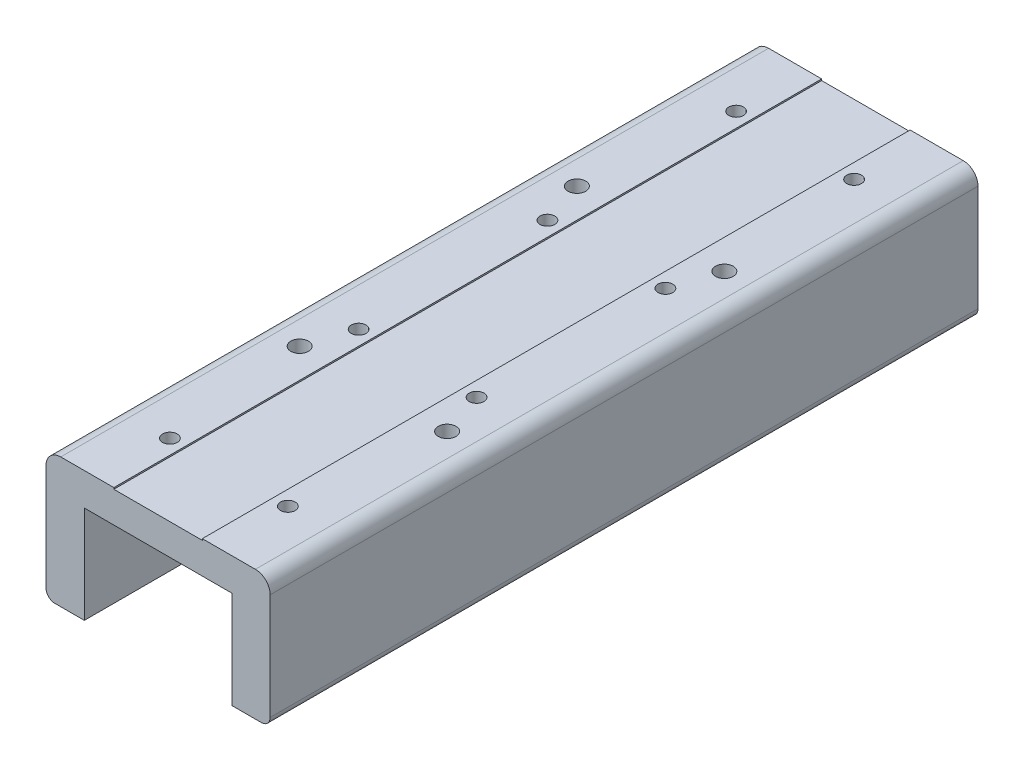
SolidWorks part; units mm, degrees
ref_plane "前视" through (0, 0, 0) normal (0, 0, 1) x (1, 0, 0)
ref_plane "上视" through (0, 0, 0) normal (0, 1, 0) x (1, 0, 0)
ref_plane "右视" through (0, 0, 0) normal (1, 0, 0) x (0, 0, -1)
sketch "草图1" plane through (0, 0, 0) normal (0, 0, 1) x (1, 0, 0)
  line L0 (0, 0) -> (0, 102.5797) construction
  line L1 (33, 50.7854) -> (15, 50.7854)
  line L2 (-38, 45.7854) -> (-38, 9.7854)
  line L3 (-35, 6.7854) -> (-25, 6.7854)
  line L4 (-25, 6.7854) -> (-25, 39.7854)
  line L5 (-25, 39.7854) -> (25, 39.7854)
  line L6 (25, 6.7854) -> (25, 39.7854)
  line L7 (35, 6.7854) -> (25, 6.7854)
  line L8 (38, 45.7854) -> (38, 9.7854)
  line L9 (-15, 50.7854) -> (-15, 50.2854)
  line L10 (-15, 50.2854) -> (15, 50.2854)
  line L11 (15, 50.7854) -> (15, 50.2854)
  line L12 (-15, 50.7854) -> (-33, 50.7854)
  arc A0 (-35, 6.7854) -> (-38, 9.7854) centre (-35, 9.7854) cw
  arc A1 (38, 9.7854) -> (35, 6.7854) centre (35, 9.7854) cw
  arc A2 (-38, 45.7854) -> (-33, 50.7854) centre (-33, 45.7854) cw
  arc A3 (38, 45.7854) -> (33, 50.7854) centre (33, 45.7854) ccw
  point P10 (0, 39.7854)
  point P13 (0, 50.7854)
  point P17 (0, 50.2854)
  point P20 (-38, 6.7854)
  point P23 (38, 6.7854)
  point P26 (-38, 50.7854)
  point P29 (38, 50.7854)
  dimension "D7" = 3
  dimension "D8" = 5
  dimension "D1" = 11
  dimension "D2" = 13
  dimension "D3" = 44
  dimension "D4" = 38
  dimension "D5" = 0.5
  dimension "D6" = 15
extrude "基体-拉伸" add sketch "草图1" against normal blind 240
ref_plane "基准面1" through (0, 0, -70) normal (0, 0, 1) x (1, 0, 0)
sketch "草图3" plane through (0, 50.7854, 0) normal (0, 1, 0) x (-1, 0, 0)
  line L0 (24.2, 0) -> (-24.2, 0) construction
  line L1 (-38, -240) -> (-38, 0) construction
  line L2 (-20, -24) -> (20, -24) construction
  line L3 (-20, -24) -> (-20, -88) construction
  line L4 (-25, -73) -> (25, -73) construction
  line L5 (-25, -73) -> (-25, -167) construction
  circle A0 centre (-20, -24) radius 2.5
  circle A1 centre (20, -24) radius 2.5
  circle A2 centre (-20, -88) radius 2.5
  circle A3 centre (20, -88) radius 2.5
  circle A4 centre (-20, -152) radius 2.5
  circle A5 centre (20, -152) radius 2.5
  circle A6 centre (-20, -216) radius 2.5
  circle A7 centre (20, -216) radius 2.5
  circle A8 centre (-25, -73) radius 3
  circle A9 centre (25, -73) radius 3
  circle A10 centre (-25, -167) radius 3
  circle A11 centre (25, -167) radius 3
  dimension "D3" = 5
  dimension "D5" = 6
  dimension "D1" = 24
  dimension "D2" = 18
  dimension "D4" = 90
  dimension "D6" = 73
  dimension "D7" = 13
  dimension "D8" = 90
extrude "切除-拉伸1" cut sketch "草图3" against normal blind 10
